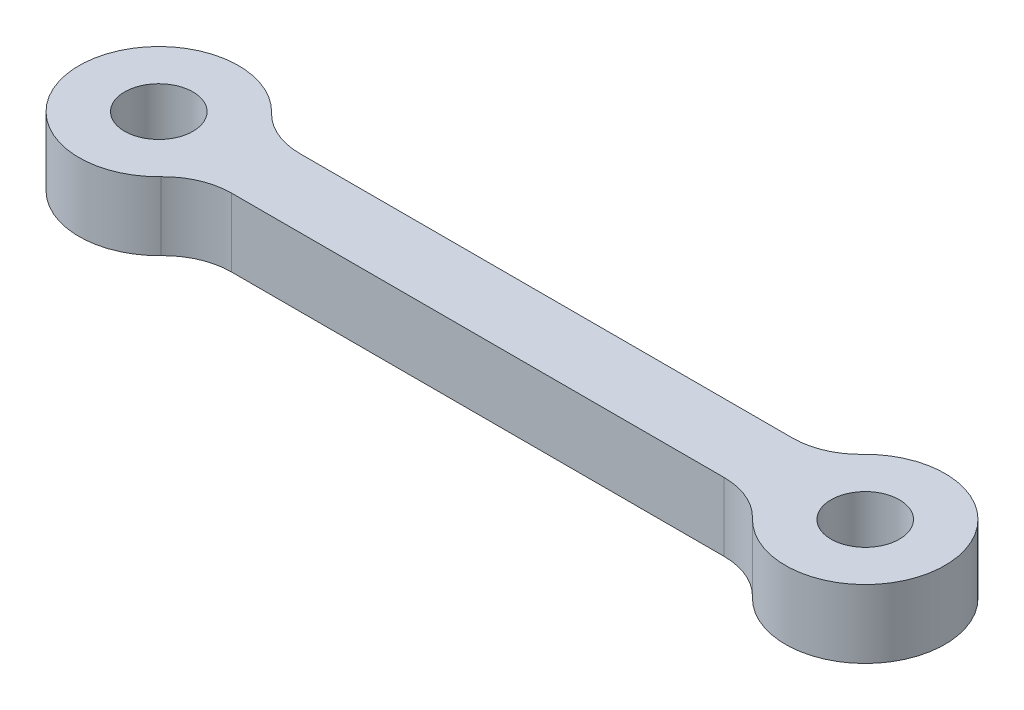
SolidWorks part; units mm, degrees
ref_plane "Front Plane" through (0, 0, 0) normal (0, 0, 1) x (1, 0, 0)
ref_plane "Top Plane" through (0, 0, 0) normal (0, 1, 0) x (1, 0, 0)
ref_plane "Right Plane" through (0, 0, 0) normal (1, 0, 0) x (0, 0, -1)
sketch "Sketch1" plane through (0, 0, 0) normal (0, 1, 0) x (1, 0, 0)
  line L0 (0, 0) -> (31, 0) construction
  line L1 (3.1623, 1.5) -> (27.8377, 1.5)
  line L2 (3.1623, -1.5) -> (27.8377, -1.5)
  circle A0 centre (0, 0) radius 3.5
  circle A1 centre (31, 0) radius 3.5
  circle A2 centre (0, 0) radius 1.5
  circle A3 centre (31, 0) radius 1.5
  dimension "D1" = 7
  dimension "D3" = 7
  dimension "D5" = 3
  dimension "D6" = 3
  dimension "D2" = 31
  dimension "D4" = 1.5
extrude "Boss-Extrude1" add sketch "Sketch1" along normal blind 3
fillet "Fillet1" radius 3 4 edges at (3.1623, 1.5, 1.5) (27.8377, 1.5, 1.5) (27.8377, 1.5, -1.5) (3.1623, 1.5, -1.5)
